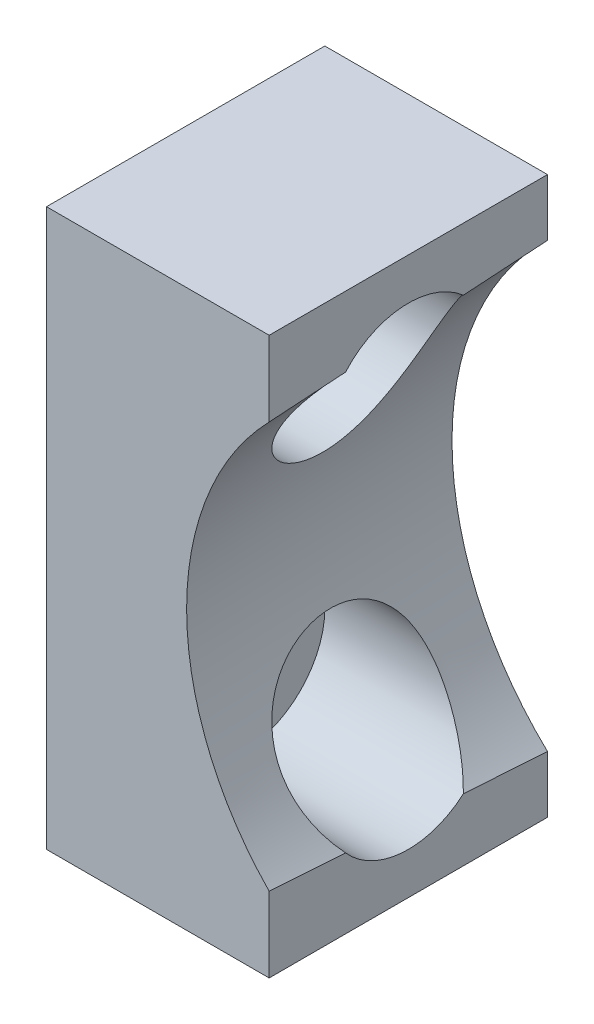
SolidWorks part; units mm, degrees
material "聚氨酯"
ref_plane "前视基准面" through (0, 0, 0) normal (0, 0, 1) x (1, 0, 0)
ref_plane "上视基准面" through (0, 0, 0) normal (0, 1, 0) x (1, 0, 0)
ref_plane "右视基准面" through (0, 0, 0) normal (1, 0, 0) x (0, 0, -1)
sketch "草图1" plane through (0, 0, 0) normal (0, 0, 1) x (1, 0, 0)
  line L1 (-4, 10) -> (4, 10)
  line L2 (-4, 10) -> (-4, -10)
  line L3 (-4, -10) -> (4, -10)
  line L4 (4, 10) -> (4, -10)
  line L5 (-4, 10) -> (4, -10) construction
  line L6 (-4, -10) -> (4, 10) construction
  point P0 (0, 0)
  dimension "D1" = 8
  dimension "D2" = 20
extrude "凸台-拉伸1" add sketch "草图1" along normal blind 10
hole_wizard "M3 六角圆柱头螺钉的柱形沉头孔1" positions "草图2" profile "草图3" counterbore size "M3" standard "GB" end condition through all
sketch "草图2" plane through (4, 0, 0) normal (1, 0, 0) x (0, 0, -1)
  line L0 (0, 0) -> (4.1737, 0) construction
  line L1 (0, -10) -> (0, 10) construction
  line L3 (-5, 10) -> (-5, 5.5) construction
  line L4 (-10, 10) -> (0, 10) construction
  point P0 (-5, 5.5)
  point P2 (-5, -5.5)
  dimension "D1" = 11
sketch "草图3" plane through (4, 5.5, 5) normal (0, 1, 0) x (0, 0, -1)
  line L0 (0, 0) -> (0, 8)
  line L1 (0, 8) -> (1.7, 8)
  line L3 (1.7, 8) -> (1.7, 6)
  line L4 (1.7, 6) -> (3, 6)
  line L5 (3, 6) -> (3, 0)
  line L7 (3, 0) -> (0, 0)
  line L11 (0, -6.35) -> (0, 107.95) construction
  dimension "通孔孔直径" = 3.4
  dimension "通孔孔深度" = 8
  dimension "柱形沉头孔直径" = 6
  dimension "柱形沉头孔深度" = 6
sketch "草图4" plane through (0, 0, 0) normal (0, 1, 0) x (1, 0, 0)
  line L0 (11.5, 1.5) -> (0.5, 1.5)
  line L1 (0.5, 1.5) -> (1.2007, -13.5817)
  line L2 (1.2007, -13.5817) -> (11.5, -13.5817)
  line L3 (11.5, -13.5817) -> (11.5, 1.5)
  line L4 (4, -10) -> (4, 0) construction
  line L5 (4, 0) -> (-4, 0) construction
  dimension "D1" = 7.5
  dimension "D2" = 11
  dimension "D3" = 87.34
  dimension "D4" = 1.5
revolve "切除-旋转1" cut sketch "草图4" angle 360 about L3
